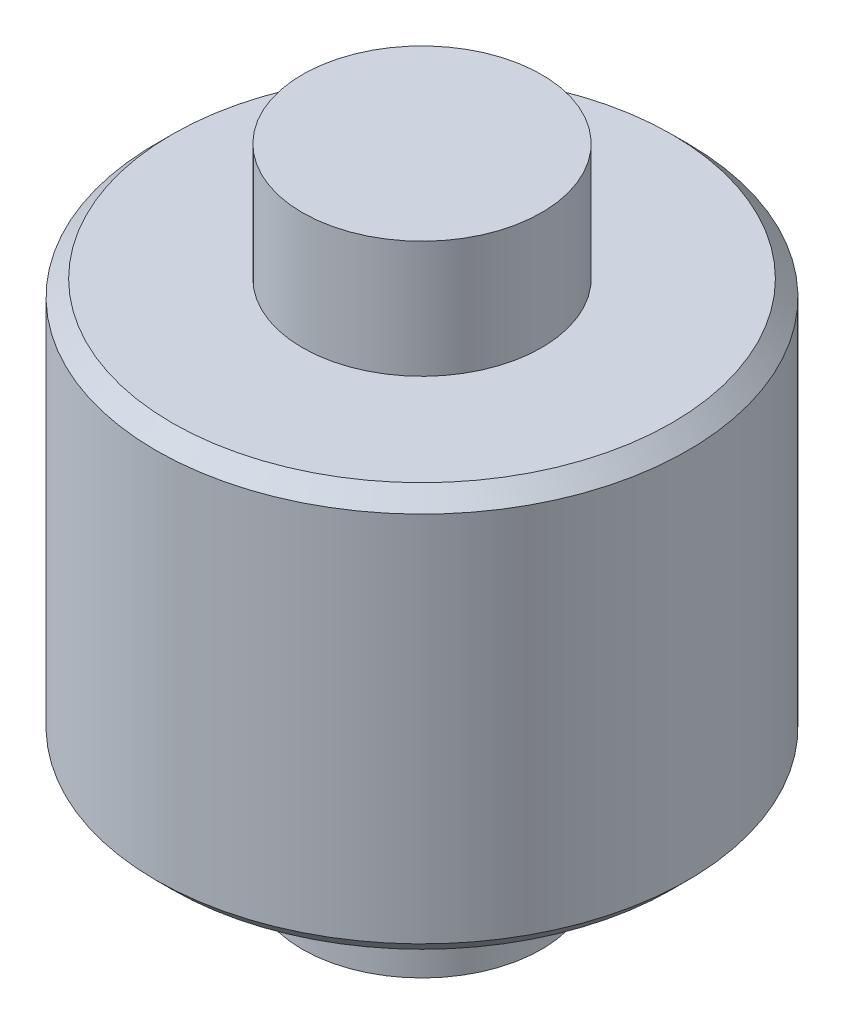
SolidWorks part; units mm, degrees
ref_plane "Front Plane" through (0, 0, 0) normal (0, 0, 1) x (1, 0, 0)
ref_plane "Top Plane" through (0, 0, 0) normal (0, 1, 0) x (1, 0, 0)
ref_plane "Right Plane" through (0, 0, 0) normal (1, 0, 0) x (0, 0, -1)
other "Configuration Table"
sketch "Sketch1" plane through (0, 0, 0) normal (0, 1, 0) x (1, 0, 0)
  circle A0 centre (0, 0) radius 45
  dimension "D1" = 90
extrude "Boss-Extrude1" add sketch "Sketch1" along normal blind 240
ref_plane "Plane1" through (0, 120, 0) normal (0, 1, 0) x (1, 0, 0)
sketch "Sketch2" plane through (0, 120, 0) normal (0, 1, 0) x (1, 0, 0)
  circle A0 centre (0, 0) radius 100
  dimension "D1" = 200
extrude "Boss-Extrude2" add sketch "Sketch2" along normal blind 76 and the other way blind 76
chamfer "Chamfer1" distance 6 angle 45 2 edges at (0, 44, 100) (0, 196, 100)
